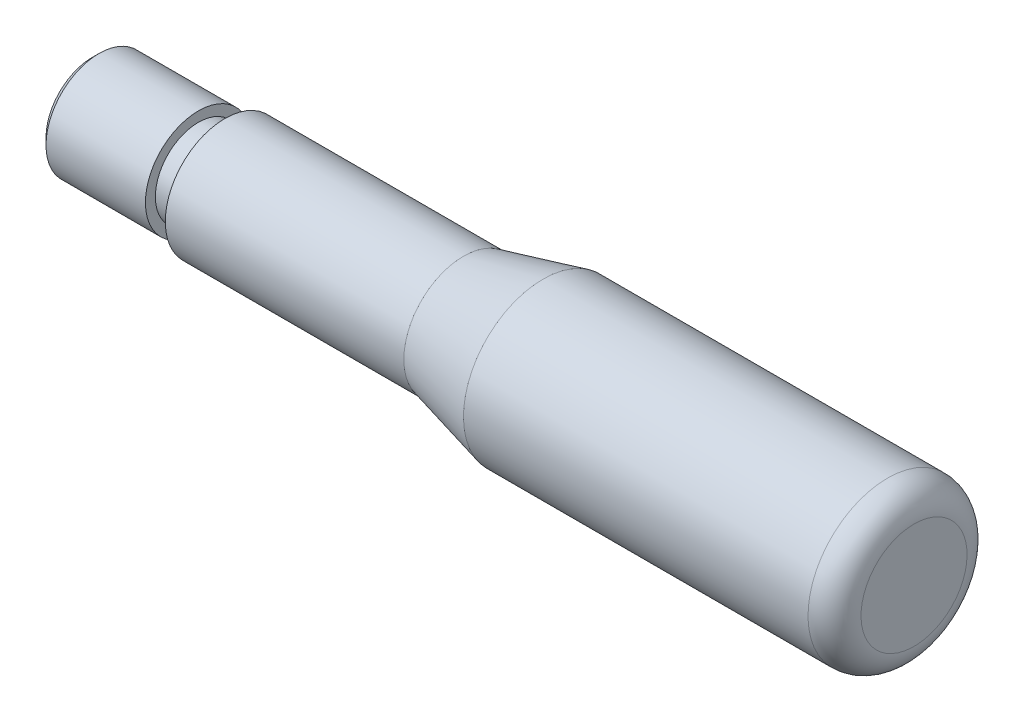
from build123d import *

# Parameters (mm, degrees)
FILLET1_R     = 2
CHAMFER1_SIZE = 0.5


with BuildPart() as part:
    # Sketch1 → Revolve1 (revolve)
    with BuildSketch(Plane.XY):
        Polygon((0, 0), (0, 4), (8, 4), (8, 3.25), (10, 3.25), (10, 4.5), (28, 4.5), (34, 6), (62, 6), (62, 0), align=None)
    revolve(axis=Axis((62, 0, 0), (-1, 0, 0)))

    # Fillet1
    fillet1_edges = [part.edges().sort_by_distance(p)[0] for p in [
        (62, -6, 0),
    ]]
    fillet(fillet1_edges, radius=FILLET1_R)

    # Chamfer1
    chamfer1_edges = [part.edges().sort_by_distance(p)[0] for p in [
        (0, -4, 0),
    ]]
    chamfer(chamfer1_edges, length=CHAMFER1_SIZE)


solid = part.part
